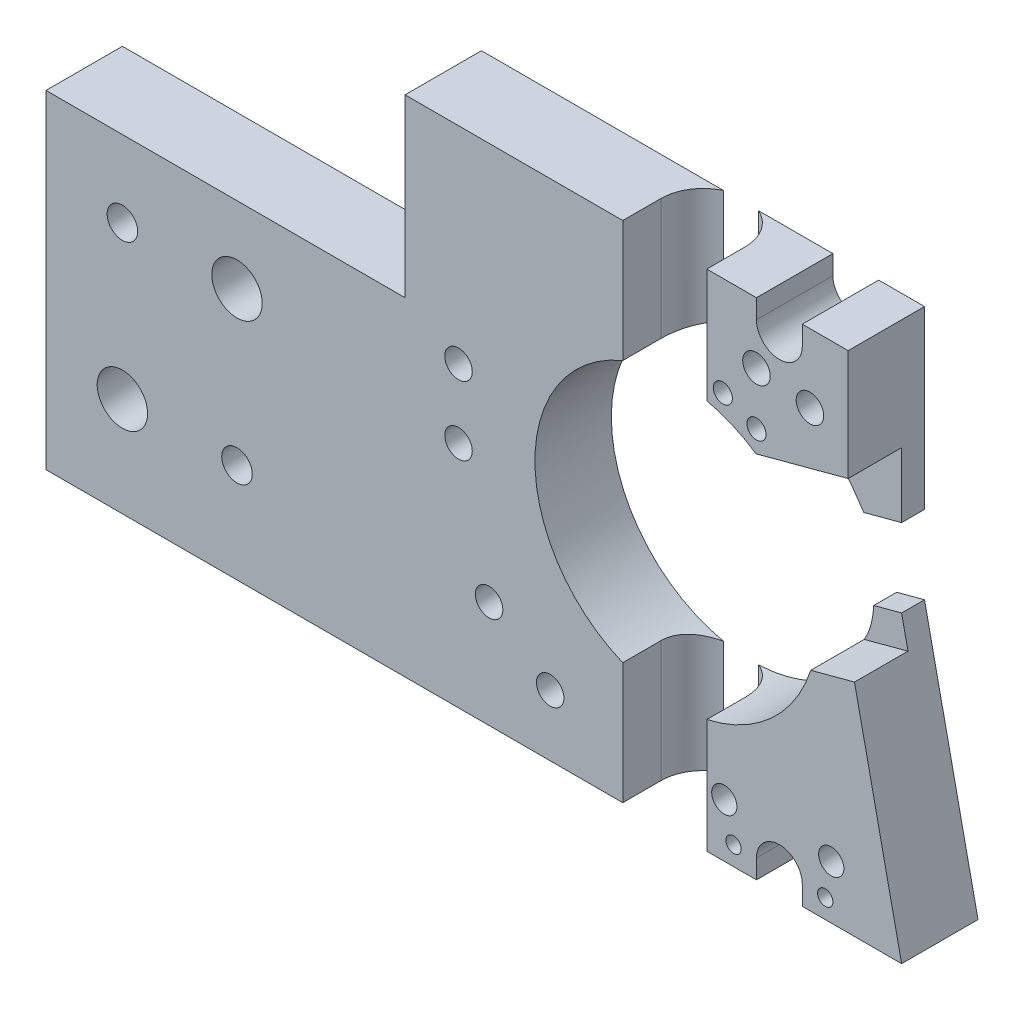
from build123d import *

# Parameters (mm, degrees)
EXTRUDE_1_DEPTH     = 10
CUT_EXTRUDE_1_DEPTH = 91.586178454
CUT_EXTRUDE_2_DEPTH = 7
CUT_EXTRUDE_3_DEPTH = 74.145140044
SKETCH_5_R          = 2
SKETCH_5_R_2        = 3.3
SKETCH_5_R_3        = 1.8
SKETCH_5_R_4        = 1.65
SKETCH_5_R_5        = 1.25
SKETCH_5_R_6        = 1
CUT_EXTRUDE_4_DEPTH = 74.145140044
CUT_EXTRUDE_5_DEPTH = 10
CUT_EXTRUDE_6_DEPTH = 10


with BuildPart() as part:
    # 草图1 → 凸台-拉伸1 (new body)
    with BuildSketch(Plane.XY):
        with BuildLine():
            Line((-50.763934426, 4.26557377), (-3.763934426, 4.26557377))
            Line((-3.763934426, 4.26557377), (-3.763934426, 27.26557377))
            Line((-3.763934426, 27.26557377), (54.236065574, 27.26557377))
            Line((54.236065574, 27.26557377), (54.236065574, 4.26557377))
            Line((54.236065574, 4.26557377), (48.224573526, 2.654799331))
            ThreePointArc((48.224573526, 2.654799331), (13.603048186, -9.400988707), (50.188626042, -7.058439882))
            Line((50.188626042, -7.058439882), (54.236065574, -5.973931728))
            Line((54.236065574, -5.973931728), (61.236065574, -38.73442623))
            Line((61.236065574, -38.73442623), (-50.763934426, -38.73442623))
            Line((-50.763934426, -38.73442623), (-50.763934426, 4.26557377))
        make_face()
    extrude(amount=EXTRUDE_1_DEPTH)

    # 草图2 → 切除-拉伸1 (cut, through all)
    with BuildSketch(Plane(origin=(0, 27.26557377, 0), x_dir=(1, 0, 0), z_dir=(0, 1, 0))):
        with BuildLine():
            Line((35.736065574, -5), (35.736065574, -10))
            Line((35.736065574, -10), (24.736065574, -10))
            Line((24.736065574, -10), (24.736065574, -5))
            ThreePointArc((24.736065574, -5), (30.236065574, 0.5), (35.736065574, -5))
        make_face()
    extrude(amount=-CUT_EXTRUDE_1_DEPTH, mode=Mode.SUBTRACT)


with BuildPart() as cut_extrude_1_piece_1:
    # of the separate pieces the step leaves, piece 1, a body of its own (cut_extrude_1_pieces)
    add(part.part.solids().sort_by_distance((-50.763934426, 4.26557377, 0))[0])


with BuildPart() as cut_extrude_1_piece_2:
    # of the separate pieces the step leaves, piece 2, a body of its own (cut_extrude_1_pieces)
    add(part.part.solids().sort_by_distance((61.236065574, -38.73442623, 0))[0])


with BuildPart() as cut_extrude_1_piece_3:
    # of the separate pieces the step leaves, piece 3, a body of its own (cut_extrude_1_pieces)
    add(part.part.solids().sort_by_distance((32.527353421, 12.748643417, 0))[0])


with BuildPart() as cut_extrude_2_tool:
    # 草图3 → 切除-拉伸2 (new body)
    with BuildSketch(Plane.XY.offset(10)):
        with BuildLine():
            Line((54.236065574, 4.26557377), (54.236065574, 12.76557377))
            Line((54.236065574, 12.76557377), (42.180479772, 9.535289291))
            ThreePointArc((42.180479772, 9.535289291), (45.635017312, 6.474961167), (48.224573526, 2.654799331))
            Line((48.224573526, 2.654799331), (54.236065574, 4.26557377))
        make_face()
        with BuildLine():
            Line((54.236065574, -5.973931728), (55.071886469, -9.885632564))
            Line((55.071886469, -9.885632564), (49.340274669, -11.421413317))
            ThreePointArc((49.340274669, -11.421413317), (49.895953848, -9.265496585), (50.188626042, -7.058439882))
            Line((50.188626042, -7.058439882), (54.236065574, -5.973931728))
        make_face()
    extrude(amount=-CUT_EXTRUDE_2_DEPTH)


with BuildPart() as cut_extrude_1_piece_2_1:
    add(cut_extrude_1_piece_2.part)

    # 切除-拉伸2: cut by cut_extrude_2_tool
    add(cut_extrude_2_tool.part, mode=Mode.SUBTRACT)


with BuildPart() as cut_extrude_1_piece_3_1:
    add(cut_extrude_1_piece_3.part)

    # 切除-拉伸2: cut by cut_extrude_2_tool
    add(cut_extrude_2_tool.part, mode=Mode.SUBTRACT)


with BuildPart() as cut_extrude_3_tool:
    # 草图4 → 切除-拉伸3 (new, through all)
    with BuildSketch(Plane.XY.offset(10)):
        with BuildLine():
            Line((42.236065574, -36.23442623), (42.236065574, -38.73442623))
            Line((42.236065574, -38.73442623), (48.236065574, -38.73442623))
            Line((48.236065574, -38.73442623), (48.236065574, -36.23442623))
            ThreePointArc((48.236065574, -36.23442623), (45.236065574, -33.23442623), (42.236065574, -36.23442623))
        make_face()
        with BuildLine():
            Line((48.236065574, 27.26557377), (42.236065574, 27.26557377))
            Line((42.236065574, 27.26557377), (42.236065574, 24.76557377))
            ThreePointArc((42.236065574, 24.76557377), (45.236065574, 21.76557377), (48.236065574, 24.76557377))
            Line((48.236065574, 24.76557377), (48.236065574, 27.26557377))
        make_face()
    extrude(amount=-CUT_EXTRUDE_3_DEPTH)


with BuildPart() as cut_extrude_1_piece_2_2:
    add(cut_extrude_1_piece_2_1.part)

    # 切除-拉伸3: cut by cut_extrude_3_tool
    add(cut_extrude_3_tool.part, mode=Mode.SUBTRACT)


with BuildPart() as cut_extrude_1_piece_3_2:
    add(cut_extrude_1_piece_3_1.part)

    # 切除-拉伸3: cut by cut_extrude_3_tool
    add(cut_extrude_3_tool.part, mode=Mode.SUBTRACT)


with BuildPart() as cut_extrude_4_tool:
    # 草图5 → 切除-拉伸4 (new, through all)
    with BuildSketch(Plane.XY.offset(10)):
        with Locations((-40.763934426, -5.73442623)):
            Circle(SKETCH_5_R)
        with Locations((-40.763934426, -25.73442623)):
            Circle(SKETCH_5_R_2)
        with Locations((-25.763934426, -5.73442623)):
            Circle(SKETCH_5_R_2)
        with Locations((-25.763934426, -25.73442623)):
            Circle(SKETCH_5_R)
        with Locations((7.236065574, -24.73442623)):
            Circle(SKETCH_5_R_3)
        with Locations((15.236065574, -30.73442623)):
            Circle(SKETCH_5_R_3)
        with Locations((3.236065574, 0.26557377)):
            Circle(SKETCH_5_R_3)
        with Locations((3.236065574, -8.73442623)):
            Circle(SKETCH_5_R_3)
        with Locations((38.027353421, -31.73442623)):
            Circle(SKETCH_5_R_4)
        with Locations((52.026065574, -31.73442623)):
            Circle(SKETCH_5_R_4)
        with Locations((42.236065574, 19.26557377)):
            Circle(SKETCH_5_R_3)
        with Locations((49.236065574, 18.26557377)):
            Circle(SKETCH_5_R_3)
        with Locations((37.836065574, 14.26557377)):
            Circle(SKETCH_5_R_5)
        with Locations((42.236065574, 12.38557377)):
            Circle(SKETCH_5_R_5)
        with Locations((39.236065574, -36.23442623)):
            Circle(SKETCH_5_R_6)
        with Locations((51.236065574, -36.23442623)):
            Circle(SKETCH_5_R_6)
    extrude(amount=-CUT_EXTRUDE_4_DEPTH)


with BuildPart() as cut_extrude_1_piece_1_1:
    add(cut_extrude_1_piece_1.part)

    # 切除-拉伸4: cut by cut_extrude_4_tool
    add(cut_extrude_4_tool.part, mode=Mode.SUBTRACT)


with BuildPart() as cut_extrude_1_piece_2_3:
    add(cut_extrude_1_piece_2_2.part)

    # 切除-拉伸4: cut by cut_extrude_4_tool
    add(cut_extrude_4_tool.part, mode=Mode.SUBTRACT)

    # 草图7 → 切除-拉伸6 (cut)
    with BuildSketch(Plane.XY.offset(3)):
        with BuildLine():
            Line((50.586440047, -6.95184594), (50.188626042, -7.058439882))
            ThreePointArc((50.188626042, -7.058439882), (49.895953848, -9.265496585), (49.340274669, -11.421413317))
            add(Edge.make_bspline(
                [(49.340274669, -11.421413317), (50.179872923, -10.066049912), (50.47464498, -8.503042836), (50.586440047, -6.95184594)],
                knots=[0, 0, 0, 0, 1, 1, 1, 1], degree=3))
        make_face()
    extrude(amount=-CUT_EXTRUDE_6_DEPTH, mode=Mode.SUBTRACT)


with BuildPart() as cut_extrude_1_piece_3_3:
    add(cut_extrude_1_piece_3_2.part)

    # 切除-拉伸4: cut by cut_extrude_4_tool
    add(cut_extrude_4_tool.part, mode=Mode.SUBTRACT)

    # 草图6 → 切除-拉伸5 (cut)
    with BuildSketch(Plane.XY.offset(3)):
        with BuildLine():
            Line((49.284985205, 2.938935784), (48.224573526, 2.654799331))
            ThreePointArc((48.224573526, 2.654799331), (45.635017312, 6.474961167), (42.180479772, 9.535289291))
            add(Edge.make_bspline(
                [(42.180479772, 9.535289291), (45.593095673, 8.546903827), (47.47999295, 5.649415813), (49.284985205, 2.938935784)],
                knots=[0, 0, 0, 0, 1, 1, 1, 1], degree=3))
        make_face()
    extrude(amount=-CUT_EXTRUDE_5_DEPTH, mode=Mode.SUBTRACT)


solid = Compound([cut_extrude_1_piece_1_1.part, cut_extrude_1_piece_2_3.part, cut_extrude_1_piece_3_3.part])
